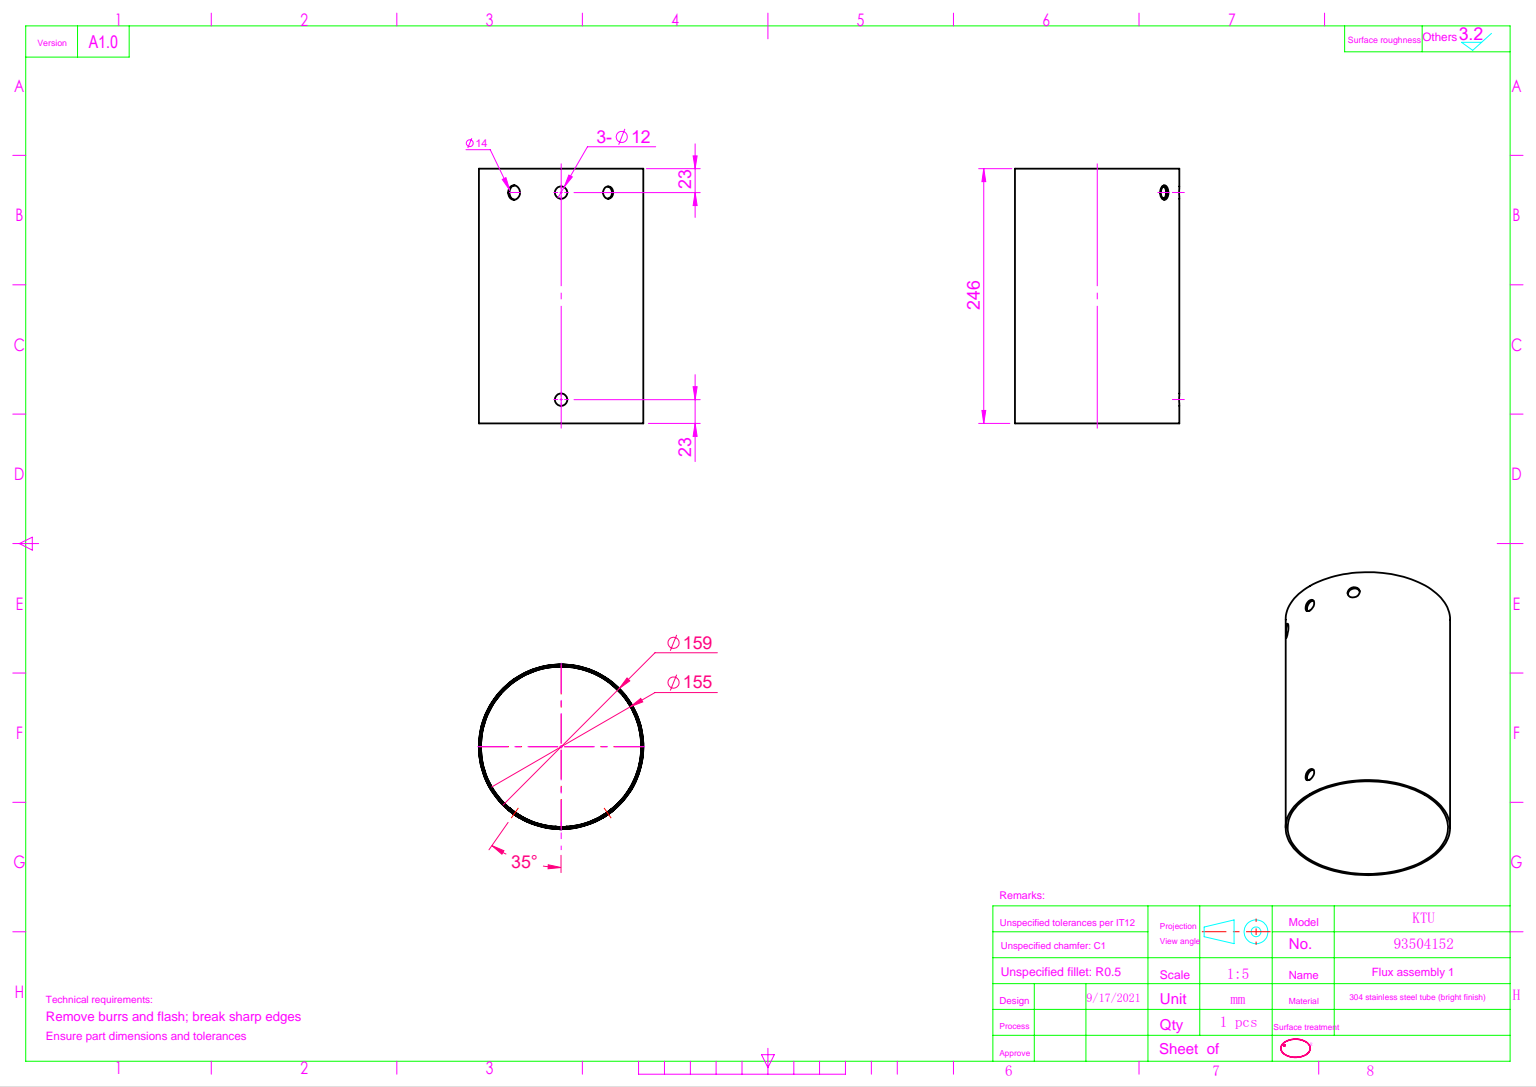
SolidWorks part; units mm, degrees
ref_plane "前视基准面" through (0, 0, 0) normal (0, 0, 1) x (1, 0, 0)
ref_plane "上视基准面" through (0, 0, 0) normal (0, 1, 0) x (1, 0, 0)
ref_plane "右视基准面" through (0, 0, 0) normal (1, 0, 0) x (0, 0, -1)
sketch "草图2" plane through (0, 0, 0) normal (0, 1, 0) x (1, 0, 0)
  circle A0 centre (0, 0) radius 79.5
  dimension "D1" = 159
extrude "拉伸-薄壁1" add sketch "草图2" along normal mid plane 246 thin thin type one direction reverse wall 2
sketch "草图3" plane through (0, 0, 0) normal (0, 0, 1) x (1, 0, 0)
  line L0 (-79.5, -123) -> (79.5, -123) construction
  circle A0 centre (0, 100) radius 6
  circle A1 centre (0, -100) radius 6
  dimension "D1" = 23
  dimension "D3" = 12
  dimension "D2" = 200
extrude "切除-拉伸2" cut sketch "草图3" along normal through all
ref_plane "基准面1" through (0, 0, 0) normal (0.5736, 0, 0.8192) x (0, -1, 0)
sketch "草图4" plane through (0, 0, 0) normal (0.5736, 0, 0.8192) x (0, -1, 0)
  line L0 (-123, 79.5) -> (-123, -79.5) construction
  circle A0 centre (-100, 0) radius 6
  dimension "D1" = 23
  dimension "D2" = 12
extrude "切除-拉伸3" cut sketch "草图4" along normal through all
ref_plane "基准面2" through (0, 0, 0) normal (0.5736, 0, -0.8192) x (0, -1, 0)
sketch "草图5" plane through (0, 0, 0) normal (0.5736, 0, -0.8192) x (0, -1, 0)
  line L0 (-123, 79.5) -> (-123, -79.5) construction
  circle A0 centre (-100, 0) radius 7
  dimension "D1" = 14
  dimension "D2" = 23
extrude "切除-拉伸4" cut sketch "草图5" against normal through all
ref_plane "基准面3" through (0, 0, 0) normal (0, 0, 1) x (0, -1, 0)
sketch "草图6" plane through (0, 0, 0) normal (0, 0, 1) x (0, -1, 0)
  line L0 (-123, 79.5) -> (-123, -79.5) construction
  circle A0 centre (-117, 0) radius 3
  dimension "D1" = 6
  dimension "D2" = 6
extrude "切除-拉伸6" [suppressed] cut sketch "草图6" along normal through all
